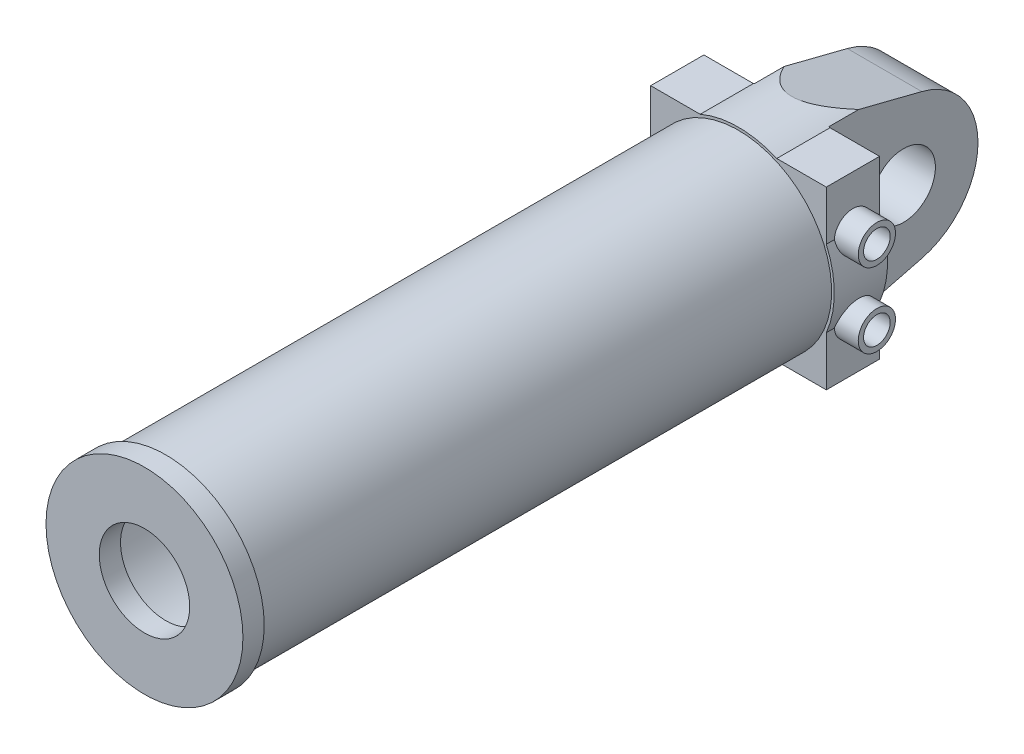
SolidWorks part; units mm, degrees
material "1.0503 (C45)"
ref_plane "前视基准面" through (0, 0, 0) normal (0, 0, 1) x (1, 0, 0)
ref_plane "上视基准面" through (0, 0, 0) normal (0, 1, 0) x (1, 0, 0)
ref_plane "右视基准面" through (0, 0, 0) normal (1, 0, 0) x (0, 0, -1)
sketch "草图1" plane through (0, 0, 0) normal (0, 0, 1) x (1, 0, 0)
  circle A0 centre (0, 0) radius 87.5
  circle A1 centre (0, 0) radius 77.5
  dimension "D1" = 175
  dimension "D2" = 10
extrude "凸台-拉伸1" add sketch "草图1" along normal blind 558
sketch "草图4" plane through (0, 0, 0) normal (0, 0, -1) x (-1, 0, 0)
  circle A0 centre (0, 0) radius 90
  dimension "D1" = 180
extrude "凸台-拉伸2" add sketch "草图4" along normal blind 50
sketch "草图5" plane through (0, 0, 0) normal (1, 0, 0) x (0, 0, -1)
  line L0 (50, 0) -> (120, 0) construction
  line L1 (50, -90) -> (50, 90) construction
  line L2 (108.625, 0) -> (-108.625, 0) construction
  line L3 (50, 90) -> (137.2308, 67.8462)
  line L4 (50, -90) -> (137.2308, -67.8462)
  line L5 (50, 90) -> (50, -90)
  circle A0 centre (120, 0) radius 30
  arc A1 (137.2308, -67.8462) -> (137.2308, 67.8462) centre (120, 0) ccw
  dimension "D1" = 60
  dimension "D2" = 140
  dimension "D3" = 70
extrude "凸台-拉伸3" add sketch "草图5" along normal mid plane 70
sketch "草图6" plane through (0, 0, -50) normal (0, 0, -1) x (-1, 0, 0)
  circle A0 centre (0, 0) radius 90
  dimension "D1" = 180
extrude "切除-拉伸2" cut sketch "草图6" along normal through all flip side to cut
sketch "草图7" plane through (0, 0, 0) normal (1, 0, 0) x (0, 0, -1)
  line L0 (0, 0) -> (50, 0) construction
  line L1 (50, 82.9156) -> (50, -82.9156) construction
  line L2 (25, 0) -> (25, 35) construction
  circle A0 centre (25, 35) radius 17.5
  circle A1 centre (25, -35) radius 17.5
  circle A2 centre (25, 35) radius 12.5
  circle A3 centre (25, -35) radius 12.5
  dimension "D1" = 35
  dimension "D2" = 70
  dimension "D3" = 5
extrude "凸台-拉伸4" add sketch "草图7" along normal blind 105
sketch "草图8" plane through (0, 0, 558) normal (0, 0, 1) x (1, 0, 0)
  circle A1 centre (0, 0) radius 42.5
  circle A2 centre (0, 0) radius 92.5
  circle A3 centre (0, 0) radius 92.5
  dimension "D1" = 5
  dimension "D2" = 85
extrude "凸台-拉伸5" add sketch "草图8" against normal blind 20
sketch "草图9" plane through (0, 0, -50) normal (0, 0, -1) x (-1, 0, 0)
  line L1 (-82.5, 82.5) -> (82.5, 82.5)
  line L2 (-82.5, 82.5) -> (-82.5, -82.5)
  line L3 (-82.5, -82.5) -> (82.5, -82.5)
  line L4 (82.5, 82.5) -> (82.5, -82.5)
  line L5 (-82.5, 82.5) -> (82.5, -82.5) construction
  line L6 (-82.5, -82.5) -> (82.5, 82.5) construction
  point P0 (0, 0)
  dimension "D1" = 165
  dimension "D2" = 165
extrude "凸台-拉伸6" add sketch "草图9" against normal blind 50
